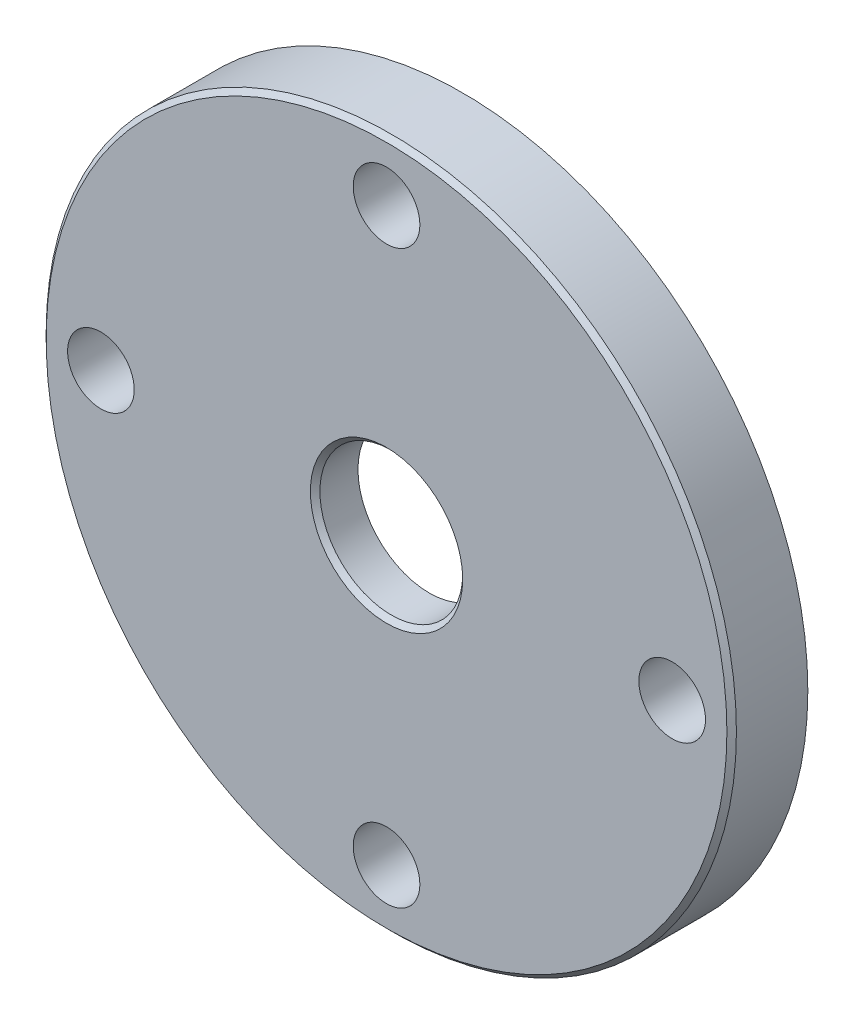
SolidWorks part; units mm, degrees
material "Q345"
ref_plane "前视基准面" through (0, 0, 0) normal (0, 0, 1) x (1, 0, 0)
ref_plane "上视基准面" through (0, 0, 0) normal (0, 1, 0) x (1, 0, 0)
ref_plane "右视基准面" through (0, 0, 0) normal (1, 0, 0) x (0, 0, -1)
sketch "草图1" plane through (0, 0, 0) normal (0, 0, 1) x (1, 0, 0)
  circle A0 centre (0, 0) radius 72.5
  dimension "D1" = 145
extrude "凸台-拉伸1" add sketch "草图1" along normal blind 16
sketch "草图2" plane through (0, 0, 16) normal (0, 0, 1) x (1, 0, 0)
  circle A0 centre (0, 0) radius 60 construction
  circle A1 centre (0, 60) radius 7
  circle A2 centre (60, 0) radius 7
  circle A3 centre (0, -60) radius 7
  circle A4 centre (-60, 0) radius 7
  point P14 (0, 0)
  dimension "D1" = 120
  dimension "D2" = 14
  dimension "D3" = 4
extrude "切除-拉伸1" cut sketch "草图2" against normal through all
sketch "草图3" plane through (0, 0, 0) normal (0, 0, -1) x (-1, 0, 0)
  circle A0 centre (0, 0) radius 46
  dimension "D1" = 92
extrude "切除-拉伸2" cut sketch "草图3" against normal blind 7
sketch "草图4" plane through (0, 0, 16) normal (0, 0, 1) x (1, 0, 0)
  circle A0 centre (0, 0) radius 15
  dimension "D1" = 30
extrude "切除-拉伸3" cut sketch "草图4" against normal through all
chamfer "倒角1" distance 1 angle 45 3 edges at (15, 0, 16) (-46, 0, 0) (72.5, 0, 16)
